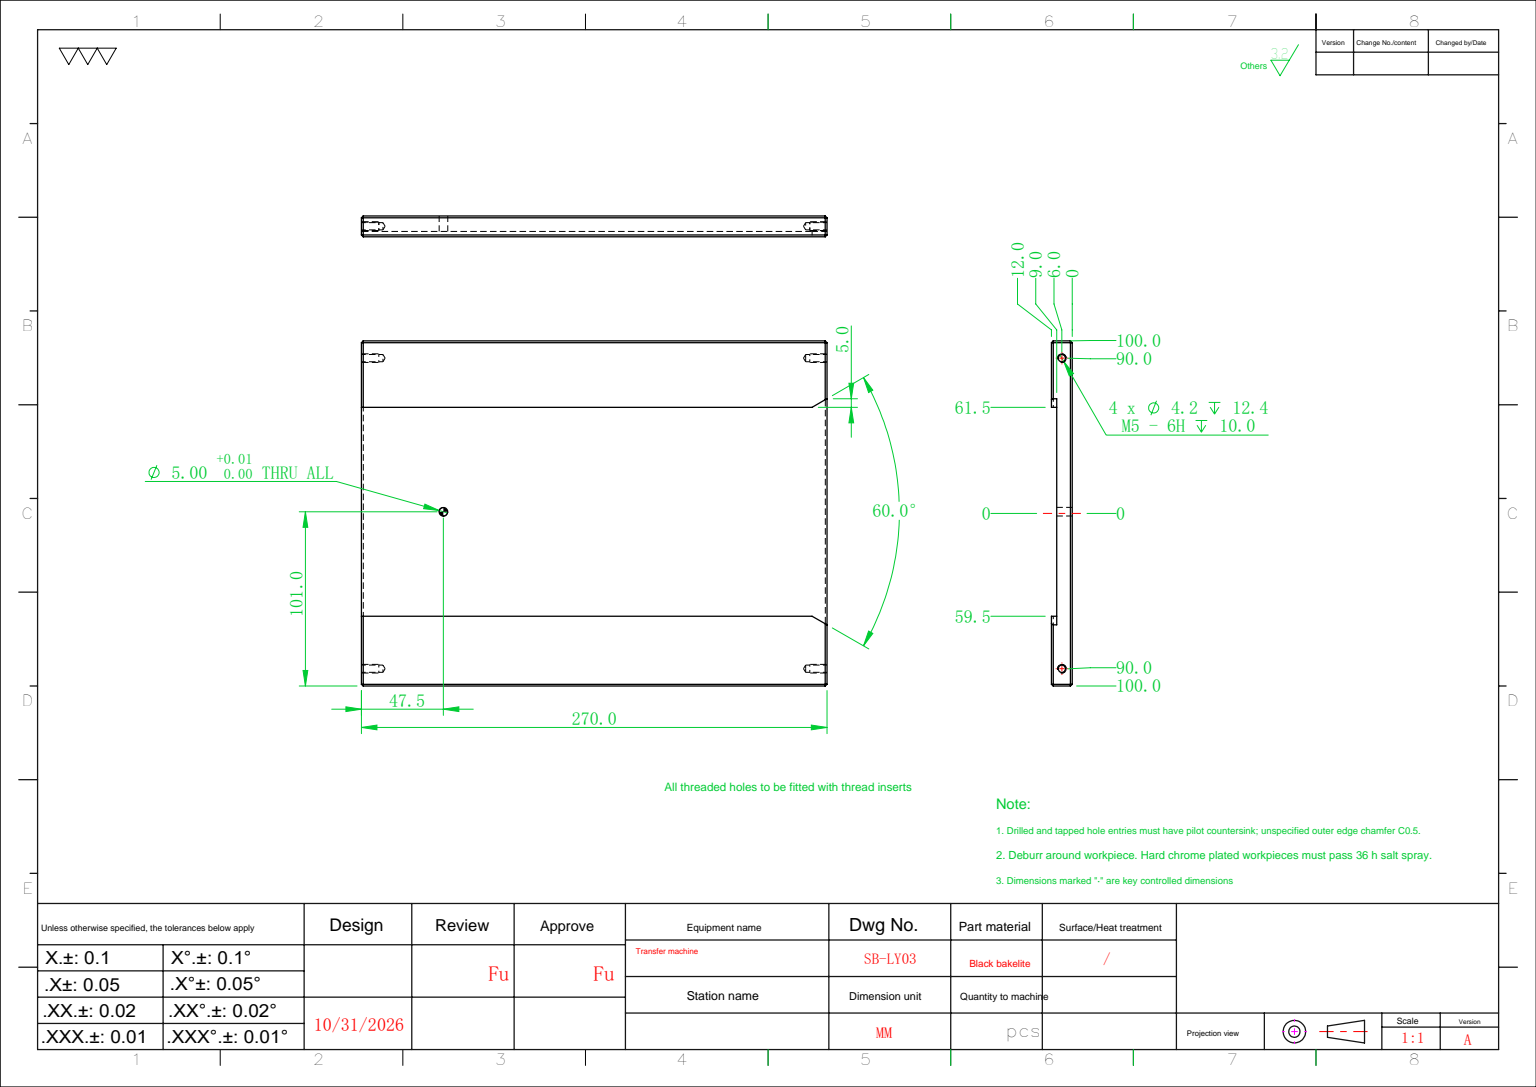
from build123d import *

# Parameters (mm, degrees)
SKETCH_1_W                  = 200
SKETCH_1_H                  = 270
EXTRUDE_1_DEPTH             = 12
SKETCH_2_W                  = 121
SKETCH_2_H                  = 270
CUT_EXTRUDE_1_DEPTH         = 3
CHAMFER_1_SIZE              = 5
CHAMFER_1_SIZE2             = 8.660254038
HOLE_WIZARD_M5_1_AT_2_COUNT = 2
HOLE_WIZARD_M5_1_AT_2_PITCH = 180
CHAMFER_2_SIZE              = 1
MM_1_D                      = 5


with BuildPart() as part:
    # 草图1 → 凸台-拉伸1 (new body)
    with BuildSketch(Plane.XY):
        Rectangle(SKETCH_1_W, SKETCH_1_H)
    extrude(amount=EXTRUDE_1_DEPTH)

    # 草图2 → 切除-拉伸1 (cut)
    with BuildSketch(Plane.XY.offset(12)):
        with Locations((-1, 0)):
            Rectangle(SKETCH_2_W, SKETCH_2_H)
    extrude(amount=-CUT_EXTRUDE_1_DEPTH, mode=Mode.SUBTRACT)

    # 倒角1
    chamfer_1_edges = [part.edges().sort_by_distance(p)[0] for p in [
        (59.5, 135, 10.5),
        (-61.5, 135, 10.5),
    ]]
    chamfer_1_side = [part.faces().sort_by_distance(p)[0] for p in [
        (0.17820324, 135, 5.19808542),
    ]]
    chamfer(chamfer_1_edges, length=CHAMFER_1_SIZE, length2=CHAMFER_1_SIZE2, reference=chamfer_1_side[0])

    # 草图4 → M5 螺纹孔1 (revolve, cut)
    with BuildSketch(Plane(origin=(90, 135, 6), x_dir=(0, 0, 1), z_dir=(1, 0, 0))):
        Polygon((0, 0), (0, 13.6618073), (2.1, 12.4), (2.1, 0), align=None)
    hole_wizard_m5_1 = revolve(axis=Axis((90, 141.35, 6), (0, -1, 0)), mode=Mode.SUBTRACT)

    # M5 螺纹孔1 at 2: M5 螺纹孔1 ×2
    with Locations(*[(-i * HOLE_WIZARD_M5_1_AT_2_PITCH, 0, 0) for i in range(1, HOLE_WIZARD_M5_1_AT_2_COUNT)]):
        add(hole_wizard_m5_1, mode=Mode.SUBTRACT)

    # 镜向1: M5 螺纹孔1 across plane
    add(hole_wizard_m5_1.mirror(Plane.ZX), mode=Mode.SUBTRACT)

    # 镜向1 copy 1 sketch → 镜向1 copy 1 (revolve, cut)
    with BuildSketch(Plane(origin=(-90, -135, 6), x_dir=(0, 0, 1), z_dir=(1, 0, 0))):
        Polygon((0, 0), (0, -13.6618073), (2.1, -12.4), (2.1, 0), align=None)
    revolve(axis=Axis((-90, -141.35, 6), (0, -1, 0)), mode=Mode.SUBTRACT)

    # 倒角2
    chamfer_2_edges = [part.edges().sort_by_distance(p)[0] for p in [
        (-100, 0, 12),
        (-80.75, -135, 12),
        (79.75, -135, 12),
        (-83.25, 135, 12),
        (100, 0, 12),
        (0, -135, 0),
        (-100, 0, 0),
        (0, 135, 0),
        (100, 0, 0),
        (82.25, 135, 12),
        (100, -135, 6),
        (-100, -135, 6),
        (-100, 135, 6),
        (100, 135, 6),
    ]]
    chamfer(chamfer_2_edges, length=CHAMFER_2_SIZE)

    # 大小mm 暗销孔1 (through all)
    with Locations(Plane.XY.offset(9)):
        with Locations((-1, -87.5)):
            Hole(MM_1_D / 2)


solid = part.part
